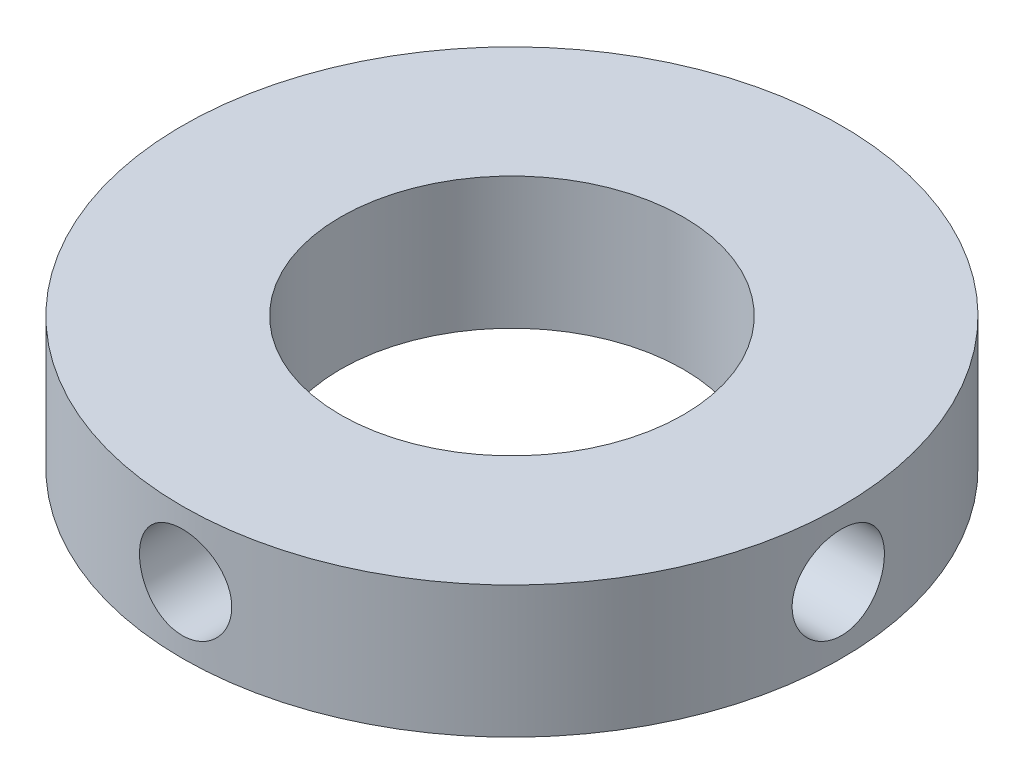
SolidWorks part; units mm, degrees
ref_plane "Front Plane" through (0, 0, 0) normal (0, 0, 1) x (1, 0, 0)
ref_plane "Top Plane" through (0, 0, 0) normal (0, 1, 0) x (1, 0, 0)
ref_plane "Right Plane" through (0, 0, 0) normal (1, 0, 0) x (0, 0, -1)
sketch "Sketch1" plane through (0, 0, 0) normal (0, 1, 0) x (1, 0, 0)
  circle A0 centre (0, 0) radius 50
  dimension "D1" = 100
extrude "Boss-Extrude1" add sketch "Sketch1" along normal blind 20
hole_wizard "M56x4.0 Tapped Hole1" positions "Sketch3" profile "Sketch4" tap size "M56x4.0" standard "GB"
sketch "Sketch3" plane through (0, 20, 0) normal (0, 1, 0) x (1, 0, 0)
  point P0 (0, 0)
sketch "Sketch4" plane through (0, 20, 0) normal (1, 0, 0) x (0, 0, 1)
  line L0 (0, 0) -> (0, 139.6224)
  line L1 (0, 139.6224) -> (26, 124)
  line L2 (26, 124) -> (26, 0)
  line L5 (26, 0) -> (0, 0)
  line L10 (0, 139.6224) -> (-26, 124) construction
  line L11 (0, -6.35) -> (0, 107.95) construction
  dimension "螺纹孔钻头直径" = 52
  dimension "螺纹孔钻头深度" = 124
  dimension "导头角度" = 118
cosmetic thread "Cosmetic Thread1" parameters "D1"=25, "D2"=56
hole_wizard "Ø14.0 (14) Diameter Hole1" positions "3DSketch1" profile "Sketch5" hole size "Ø14.0" standard "GB"
sketch3d "3DSketch1"
  line L0 (0, 0, 0) -> (0, 0, 50) construction
  line L1 (0, 0, 50) -> (0, 20, 50) construction
  circle A0 centre (0, 0, 0) radius 50 construction
  circle A1 centre (0, 20, 0) radius 50 construction
  point P0 (0, 10, 50)
  point P8 (0, 50, 0)
  point P12 (0, 70, 0)
sketch "Sketch5" plane through (0, 10, 50) normal (1, 0, 0) x (0, -1, 0)
  line L0 (0, 0) -> (0, 20)
  line L1 (0, 20) -> (7, 15.794)
  line L2 (7, 15.794) -> (7, 0)
  line L5 (7, 0) -> (0, 0)
  line L10 (0, 20) -> (-7, 15.794) construction
  line L11 (0, -6.35) -> (0, 107.95) construction
  dimension "孔直径" = 14
  dimension "孔深度" = 20
  dimension "导头角度" = 118
pattern_circular "CirPattern1" count 4 over 360 about axis through (0, 20, 0) along (0, 1, 0) of "Ø14.0 (14) Diameter Hole1"
